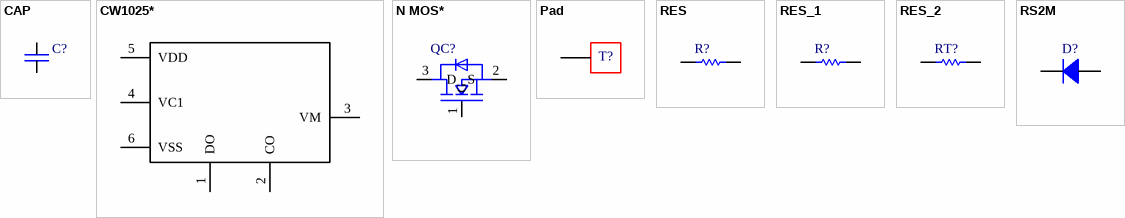
[diagram p0: symbols CAP to RS2M]
# Altium schematic symbol library MISC82114.SCHLIB: 8 symbols
Pins are listed as number, name and electrical type; pins without a type are passive.


## CAP
designator C?
SMD capacitor
footprint C0402A (SMD capacitor)
footprint C0603A (SMD capacitor)
footprint C0402L (SMD resistor)
footprint C0805A (SMD capacitor)
footprint C1206A (SMD capacitor)
footprint C0603L (SMD J capacitor)
footprint C0805L (SMD capacitor)
footprint C0603M (SMD capacitor)
pins: 1, 2

## CW1025*
designator U?
1-2S battery protection IC
footprint SOT-23-6
footprint SOT23-6A
pins: 1 DO, 2 CO, 3 VM, 4 VC1, 5 VDD, 6 VSS

## N MOS*
designator QC?
SMD MOSFET
footprint TO-252
footprint TO-252-DFN
footprint SOP-8L(T3p)
footprint DFN5X6(T3p) (SMD MOSFET (non-standard))
footprint TO-263-TOLL
footprint DFN-3x3L8(T3P) (SMD MOSFET)
footprint TOLL_123 (SMD MOSFET)
footprint TOLL_GSD (SMD MOSFET)
pins: 1 G, 2 S, 3 D

## Pad
designator T?
Connection pad (non-through-hole)
footprint 3*3
footprint Pad10X8mm
footprint Pad8X6mm
pins: 1

## RES
designator R?
SMD resistor
footprint R0603A (SMD resistor)
footprint R0201A
footprint R0402A (SMD resistor)
footprint R0603m (SMD resistor)
footprint R0805A (SMD resistor)
footprint R0402L (SMD resistor)
footprint RES0603 (CAP0402)
footprint R0603L (SMD resistor)
footprint R0805L (SMD resistor)
footprint R0805M (SMD resistor)
footprint R1206A (SMD resistor)
pins: 1, 2

## RES_1
designator R?
SMD resistor
footprint R0603A (SMD resistor)
footprint R0201A
footprint R0402A (SMD resistor)
footprint R0603m (SMD resistor)
footprint R0805A (SMD resistor)
footprint R0402L (SMD resistor)
footprint RES0603 (CAP0402)
footprint R0603L (SMD resistor)
footprint R0805L (SMD resistor)
footprint R0805M (SMD resistor)
footprint R1206A (SMD resistor)
pins: 1, 2

## RES_2
designator RT?
SMD resistor
footprint R0603A (SMD resistor)
footprint R0201A
footprint R0402A (SMD resistor)
footprint R0603m (SMD resistor)
footprint R0805A (SMD resistor)
footprint R0402L (SMD resistor)
footprint RES0603 (CAP0402)
footprint R0603L (SMD resistor)
footprint R0805L (SMD resistor)
footprint R0805M (SMD resistor)
footprint R1206A (SMD resistor)
pins: 1, 2

## RS2M
designator D?
SMD diode
footprint SMA(DO-214AC) (SMD diode)
footprint SMB(DO-214AA) (SMD diode)
pins: 1 A, 2 K